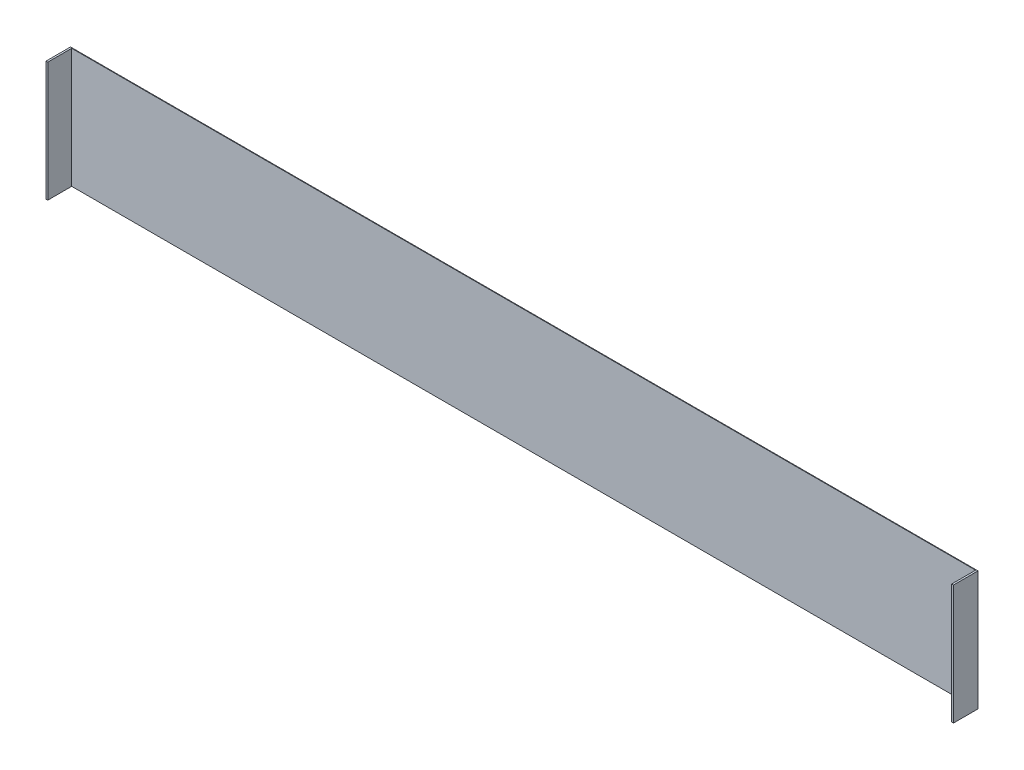
from build123d import *

# Parameters (mm, degrees)
SKETCH_1_W      = 1518
SKETCH_1_H      = 200
EXTRUDE_1_DEPTH = 1
SKETCH_2_W      = 3
SKETCH_2_H      = 200
EXTRUDE_2_DEPTH = 40


with BuildPart() as part:
    # 草图1 → 凸台-拉伸1 (new body)
    with BuildSketch(Plane.XY):
        Rectangle(SKETCH_1_W, SKETCH_1_H)
    extrude(amount=EXTRUDE_1_DEPTH)

    # 草图2 → 凸台-拉伸2 (add)
    with BuildSketch(Plane.XY.offset(1)):
        with Locations((-757.5, 0)):
            Rectangle(SKETCH_2_W, SKETCH_2_H)
    extrude_2 = extrude(amount=EXTRUDE_2_DEPTH)

    # 镜向1: 凸台-拉伸2 across plane
    add(extrude_2.mirror(Plane(origin=(0, 0, 0), x_dir=(0, 0, 1), z_dir=(1, 0, 0))))


solid = part.part
